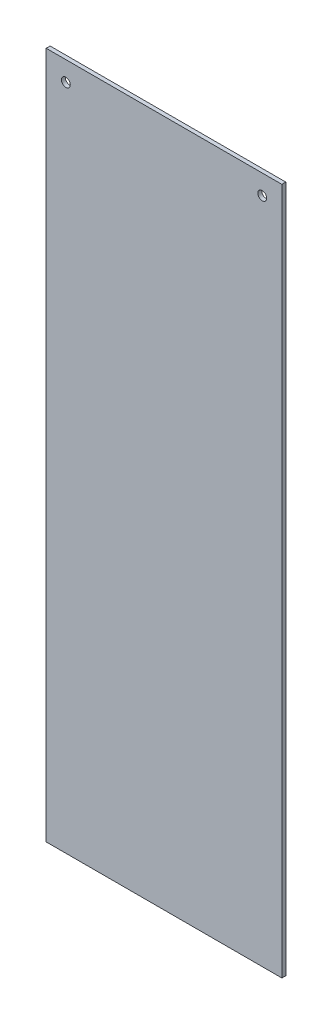
from build123d import *

# Parameters (mm, degrees)
SKETCH_1_W          = 120
SKETCH_1_H          = 350
EXTRUDE_1_DEPTH     = 2
SKETCH_2_R          = 2.25
CUT_EXTRUDE_1_DEPTH = 10


with BuildPart() as part:
    # 草图1 → 凸台-拉伸1 (new body)
    with BuildSketch(Plane.XY):
        Rectangle(SKETCH_1_W, SKETCH_1_H)
    extrude(amount=EXTRUDE_1_DEPTH)

    # 草图2 → 切除-拉伸1 (cut)
    with BuildSketch(Plane.XY.offset(2)):
        with Locations((-50, 165)):
            Circle(SKETCH_2_R)
        with Locations((50, 165)):
            Circle(SKETCH_2_R)
    extrude(amount=-CUT_EXTRUDE_1_DEPTH, mode=Mode.SUBTRACT)


solid = part.part
